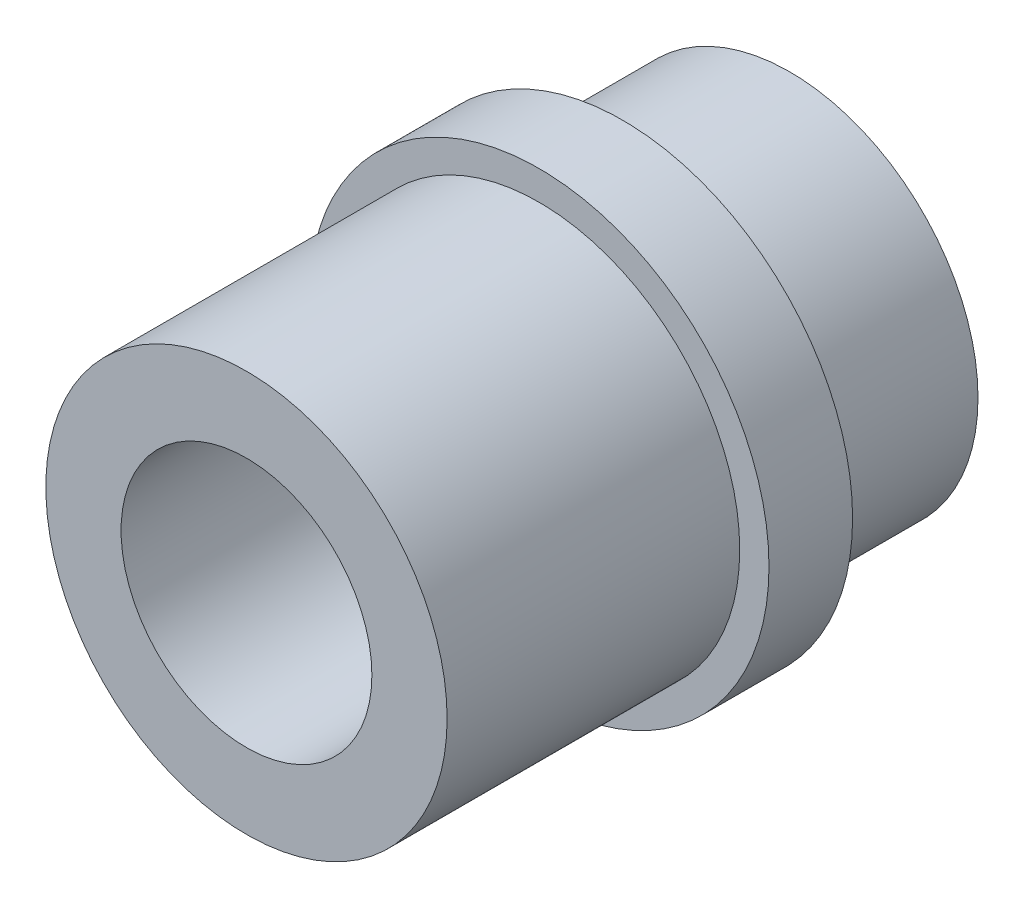
SolidWorks part; units mm, degrees
material "Q235B"
ref_plane "Front Plane" through (0, 0, 0) normal (0, 0, 1) x (1, 0, 0)
ref_plane "Top Plane" through (0, 0, 0) normal (0, 1, 0) x (1, 0, 0)
ref_plane "Right Plane" through (0, 0, 0) normal (1, 0, 0) x (0, 0, -1)
sketch "Sketch1" plane through (0, 0, 0) normal (0, 1, 0) x (1, 0, 0)
  line L0 (0, 0) -> (0, 21.798) construction
  line L1 (15, 0) -> (24, 0)
  line L2 (24, 0) -> (24, 35)
  line L3 (24, 35) -> (27.5, 35)
  line L4 (27.5, 35) -> (27.5, 45)
  line L5 (27.5, 45) -> (22.5, 45)
  line L6 (22.5, 45) -> (22.5, 65)
  line L7 (22.5, 65) -> (12.5, 65)
  line L8 (12.5, 65) -> (12.5, 30)
  line L9 (12.5, 30) -> (15, 30)
  line L10 (15, 30) -> (15, 0)
  dimension "D1" = 30
  dimension "D2" = 25
  dimension "D3" = 35
  dimension "D4" = 65
  dimension "D5" = 10
  dimension "D6" = 30
  dimension "D7" = 48
  dimension "D8" = 55
  dimension "D9" = 45
revolve "Revolve1" add sketch "Sketch1" angle 360 about L0
cosmetic thread "Cosmetic Thread1" parameters "D1"=23, "D2"=42.587
hole_wizard "M30x2.0 Tapped Hole1" positions "Sketch2" profile "Sketch3" tap size "M30x2.0" standard "GB"
sketch "Sketch2" plane through (0, 0, -65) normal (0, 0, -1) x (-1, 0, 0)
  point P0 (0, 0)
sketch "Sketch3" plane through (0, 0, -65) normal (1, 0, 0) x (0, 1, 0)
  line L0 (0, 0) -> (0, 43.412)
  line L1 (0, 43.412) -> (14, 35)
  line L2 (14, 35) -> (14, 0)
  line L5 (14, 0) -> (0, 0)
  line L10 (0, 43.412) -> (-14, 35) construction
  line L11 (0, -6.35) -> (0, 107.95) construction
  dimension "螺纹孔钻头直径" = 28
  dimension "螺纹孔钻头深度" = 35
  dimension "导头角度" = 118
cosmetic thread "Hole thread 1"
